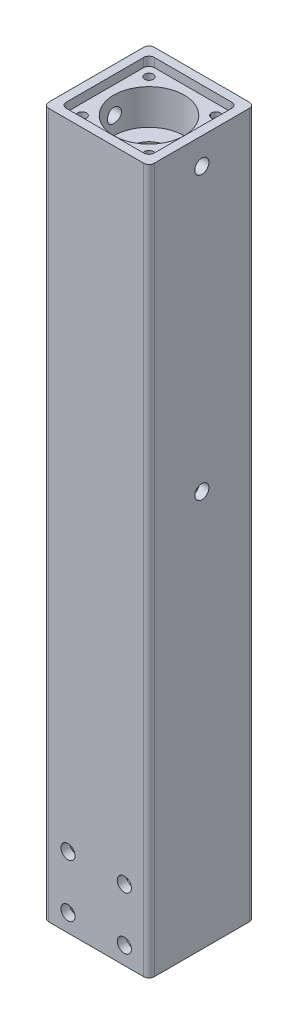
SolidWorks part; units mm, degrees
ref_plane "Front Plane" through (0, 0, 0) normal (0, 0, 1) x (1, 0, 0)
ref_plane "Top Plane" through (0, 0, 0) normal (0, 1, 0) x (1, 0, 0)
ref_plane "Right Plane" through (0, 0, 0) normal (1, 0, 0) x (0, 0, -1)
other "Configuration Table"
sketch "Sketch1" plane through (0, 0, 0) normal (0, 1, 0) x (1, 0, 0)
  line L1 (-30, 30) -> (30, 30)
  line L2 (-30, 30) -> (-30, -30)
  line L3 (-30, -30) -> (30, -30)
  line L4 (30, 30) -> (30, -30)
  line L5 (-30, 30) -> (30, -30) construction
  line L6 (-30, -30) -> (30, 30) construction
  point P0 (0, 0)
  dimension "D1" = 60
  dimension "D2" = 60
extrude "Boss-Extrude1" add sketch "Sketch1" along normal blind 400 contours L2 L3 L4 L1
sketch "Sketch2" plane through (0, 400, 0) normal (0, 1, 0) x (1, 0, 0)
  line L1 (-25, 25) -> (25, 25)
  line L2 (-25, 25) -> (-25, -25)
  line L3 (-25, -25) -> (25, -25)
  line L4 (25, 25) -> (25, -25)
  line L5 (-25, 25) -> (25, -25) construction
  line L6 (-25, -25) -> (25, 25) construction
  point P1 (0, 0)
  dimension "D1" = 50
  dimension "D2" = 50
extrude "Cut-Extrude1" cut sketch "Sketch2" against normal blind 5
sketch "Sketch3" plane through (0, 395, 0) normal (0, 1, 0) x (1, 0, 0)
  circle A0 centre (0, 0) radius 20
  dimension "D1" = 40
extrude "Cut-Extrude2" cut sketch "Sketch3" against normal blind 20
sketch "Sketch4" plane through (0, 375, 0) normal (0, 1, 0) x (1, 0, 0)
  circle A0 centre (0, 0) radius 10
  dimension "D1" = 20
extrude "Cut-Extrude3" cut sketch "Sketch4" against normal blind 15
fillet "Fillet1" radius 3 4 edges at (30, 200, 30) (-30, 200, 30) (30, 200, -30) (-30, 200, -30)
sketch "Sketch5" plane through (0, 0, 0) normal (1, 0, 0) x (0, 0, -1)
  circle A0 centre (0, 385) radius 4
  dimension "D2" = 8
extrude "Cut-Extrude4" cut sketch "Sketch5" against normal blind 30 and the other way blind 30
sketch "Sketch6" plane through (0, 0, 0) normal (0, -1, 0) x (1, 0, 0)
  line L1 (-25, 25) -> (25, 25)
  line L2 (-25, 25) -> (-25, -25)
  line L3 (-25, -25) -> (25, -25)
  line L4 (25, 25) -> (25, -25)
  line L5 (-25, 25) -> (25, -25) construction
  line L6 (-25, -25) -> (25, 25) construction
  point P0 (0, 0)
  dimension "D1" = 50
  dimension "D2" = 50
extrude "Cut-Extrude5" cut sketch "Sketch6" against normal blind 60
sketch "Sketch7" plane through (0, 60, 0) normal (0, -1, 0) x (1, 0, 0)
  circle A0 centre (0, 0) radius 25
  dimension "D1" = 50
extrude "Cut-Extrude6" cut sketch "Sketch7" against normal blind 300
sketch "Sketch8" plane through (0, 0, 0) normal (1, 0, 0) x (0, 0, -1)
  circle A0 centre (0, 225) radius 4
  dimension "D2" = 8
extrude "Cut-Extrude7" cut sketch "Sketch8" against normal blind 30 and the other way blind 30
sketch "Sketch10" plane through (0, 0, 0) normal (0, 0, 1) x (1, 0, 0)
  line L0 (0, 0) -> (0, 25)
  circle A0 centre (-16, 40) radius 4
  circle A1 centre (-16, 10) radius 4
  circle A2 centre (16, 10) radius 4
  circle A3 centre (16, 40) radius 4
  dimension "D4" = 8
  dimension "D5" = 8
  dimension "D1" = 25
  dimension "D2" = 30
  dimension "D3" = 32
extrude "Cut-Extrude9" cut sketch "Sketch10" against normal blind 30 and the other way blind 30 contours A0 | A1 | A3 | A2
fillet "Fillet2" radius 3 4 edges at (-25, 397.5, 25) (-25, 397.5, -25) (25, 397.5, 25) (25, 397.5, -25)
sketch "Sketch11" plane through (0, 395, 0) normal (0, 1, 0) x (1, 0, 0)
  circle A0 centre (-19, 19) radius 2.5
  circle A1 centre (19, 19) radius 2.5
  circle A2 centre (-19, -19) radius 2.5
  circle A3 centre (19, -19) radius 2.5
  point P0 (0, 0)
  dimension "D3" = 5
  dimension "D4" = 5
  dimension "D5" = 5
  dimension "D6" = 5
  dimension "D1" = 38
  dimension "D2" = 38
extrude "Cut-Extrude11" cut sketch "Sketch11" against normal blind 20
